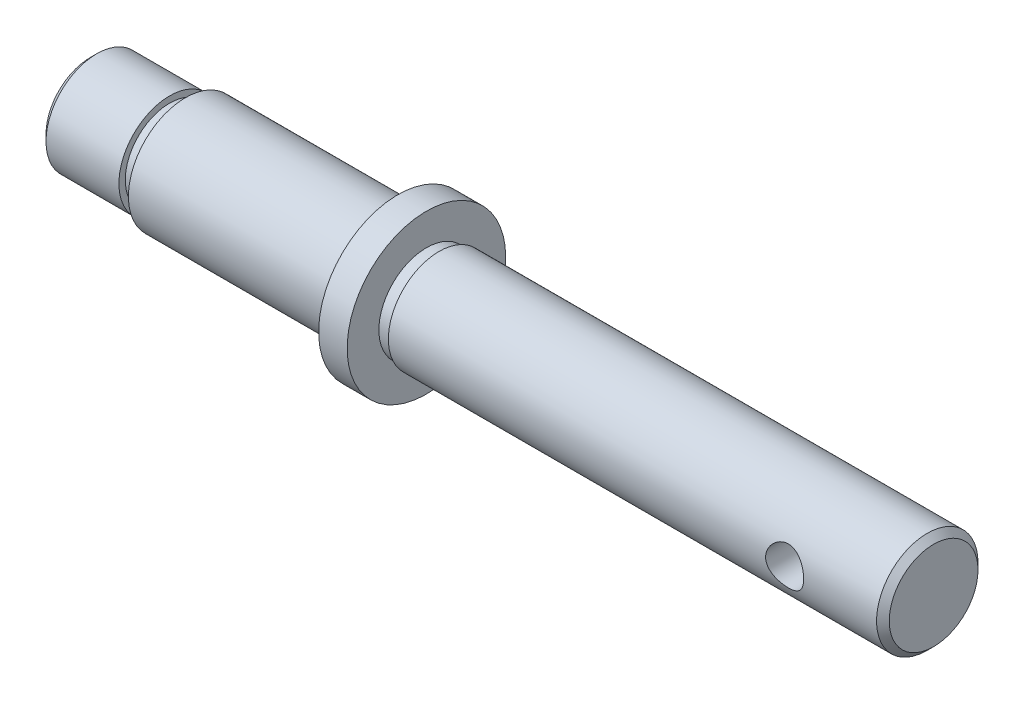
from build123d import *

# Parameters (mm, degrees)
CUT_EXTRUDE1_DEPTH      = 135.169668703
CUT_EXTRUDE1_DEPTH_BACK = 135.169668703
SKETCH2_R               = 3
CUT_EXTRUDE2_DEPTH      = 135.169668803
CUT_EXTRUDE2_DEPTH_BACK = 8
SKETCH3_R               = 3
SKETCH4_R               = 1.5
CUT_EXTRUDE3_DEPTH      = 50
CHAMFER1_SIZE           = 1.5
CHAMFER1_SIZE2          = 0.866025404
CHAMFER2_SIZE           = 1


with BuildPart() as part:
    # Sketch1 → Revolve1 (revolve)
    with BuildSketch(Plane.XY, mode=Mode.PRIVATE) as revolve1_sk:
        Polygon((0, 0), (0, 8), (12.5, 8), (12.5, 7), (15, 7), (15, 9), (46.5, 9), (46.5, 8.5), (48.5, 8.5), (48.5, 12.5), (53, 12.5), (53, 7.5), (55, 7.5), (55, 8), (133, 8), (133, 0), align=None)
    revolve(revolve1_sk.sketch.rotate(Axis((133, 0, 0), (-1, 0, 0)), 90), axis=Axis((133, 0, 0), (-1, 0, 0)))

    # Sketch2 → Cut-Extrude1 (cut, two sides: drawn at the far end of the back side and taken through both)
    with BuildSketch(Plane.XY.offset(-CUT_EXTRUDE1_DEPTH_BACK)):
        with Locations((117.5, 0)):
            Circle(SKETCH2_R)
    extrude(amount=CUT_EXTRUDE1_DEPTH + CUT_EXTRUDE1_DEPTH_BACK, mode=Mode.SUBTRACT)

    # Sketch3 → Cut-Extrude2 (cut, two sides: drawn at the far end of the back side and taken through both)
    with BuildSketch(Plane.ZY.offset(-CUT_EXTRUDE2_DEPTH_BACK)):
        with Locations(Location((0, 0, 0), (0, 0, 180))):
            Circle(SKETCH3_R)
    extrude(amount=CUT_EXTRUDE2_DEPTH + CUT_EXTRUDE2_DEPTH_BACK, mode=Mode.SUBTRACT)

    # Sketch4 → Cut-Extrude3 (cut)
    with BuildSketch(Plane.ZY.offset(-8)):
        Circle(SKETCH4_R)
    extrude(amount=-CUT_EXTRUDE3_DEPTH, mode=Mode.SUBTRACT)

    # Chamfer1
    chamfer1_edges = [part.edges().sort_by_distance(p)[0] for p in [
        (0, 0, 3),
    ]]
    chamfer1_side = [part.faces().sort_by_distance(p)[0] for p in [
        (4, 0, 3),
    ]]
    chamfer(chamfer1_edges, length=CHAMFER1_SIZE, length2=CHAMFER1_SIZE2, reference=chamfer1_side[0])

    # Chamfer2
    chamfer2_edges = [part.edges().sort_by_distance(p)[0] for p in [
        (133, 0, 8),
        (0, 0, 8),
    ]]
    chamfer(chamfer2_edges, length=CHAMFER2_SIZE)

    # Sketch5 → Cut-Revolve1 (revolve, cut)
    with BuildSketch(Plane.XY):
        with BuildLine():
            Line((58, 1.5), (58, -1.5))
            ThreePointArc((58, -1.5), (59.5, 0), (58, 1.5))
        make_face()
    revolve(axis=Axis((58, 1.5, 0), (0, -1, 0)), mode=Mode.SUBTRACT)


solid = part.part
